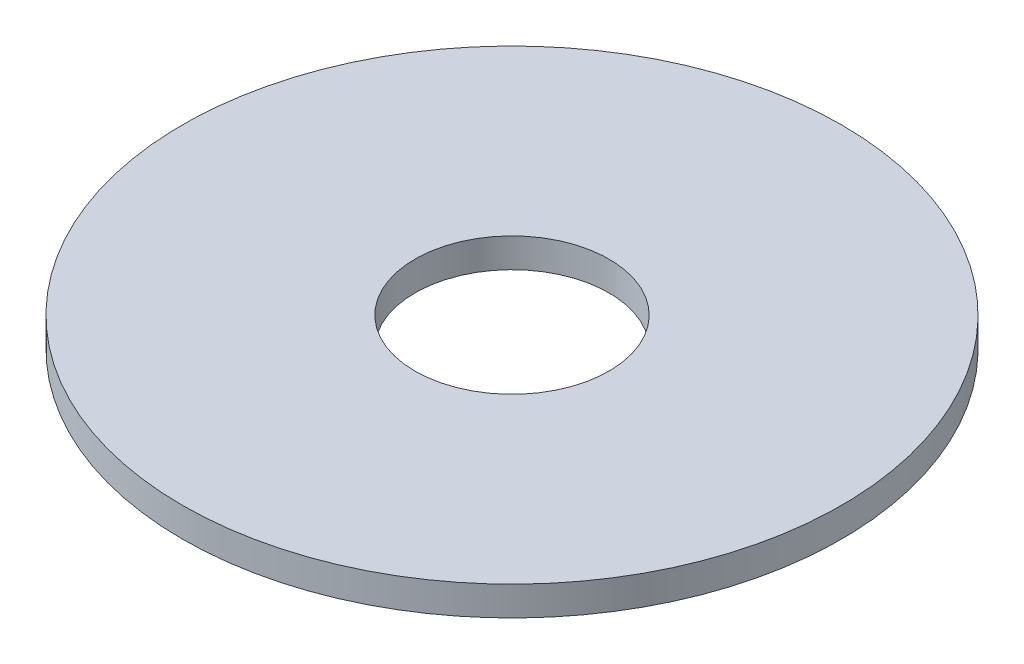
SolidWorks part; units mm, degrees
ref_plane "前视基准面" through (0, 0, 0) normal (0, 0, 1) x (1, 0, 0)
ref_plane "上视基准面" through (0, 0, 0) normal (0, 1, 0) x (1, 0, 0)
ref_plane "右视基准面" through (0, 0, 0) normal (1, 0, 0) x (0, 0, -1)
sketch "草图1" plane through (0, 0, 0) normal (0, 1, 0) x (1, 0, 0)
  circle A0 centre (0, 0) radius 13.25
  circle A1 centre (0, 0) radius 45
  dimension "D1" = 26.5
  dimension "D2" = 90
extrude "凸台-拉伸1" add sketch "草图1" along normal mid plane 4
sketch "草图2" plane through (0, -2, 0) normal (0, -1, 0) x (1, 0, 0)
  line L0 (-13.2384, 0.5547) -> (-13.2384, 3.5547)
  line L1 (13.2384, 0.5547) -> (13.2384, 3.5547)
  line L2 (-13.2384, 0.5547) -> (13.2384, 0.5547)
  circle A0 centre (0, 0) radius 13.25 construction
  arc A1 (13.2384, 3.5547) -> (-13.2384, 3.5547) centre (0, 15) ccw
  dimension "D1" = 35
  dimension "D2" = 3
  dimension "D3" = 15
extrude "切除-拉伸1" [suppressed] cut sketch "草图2" against normal up to next
